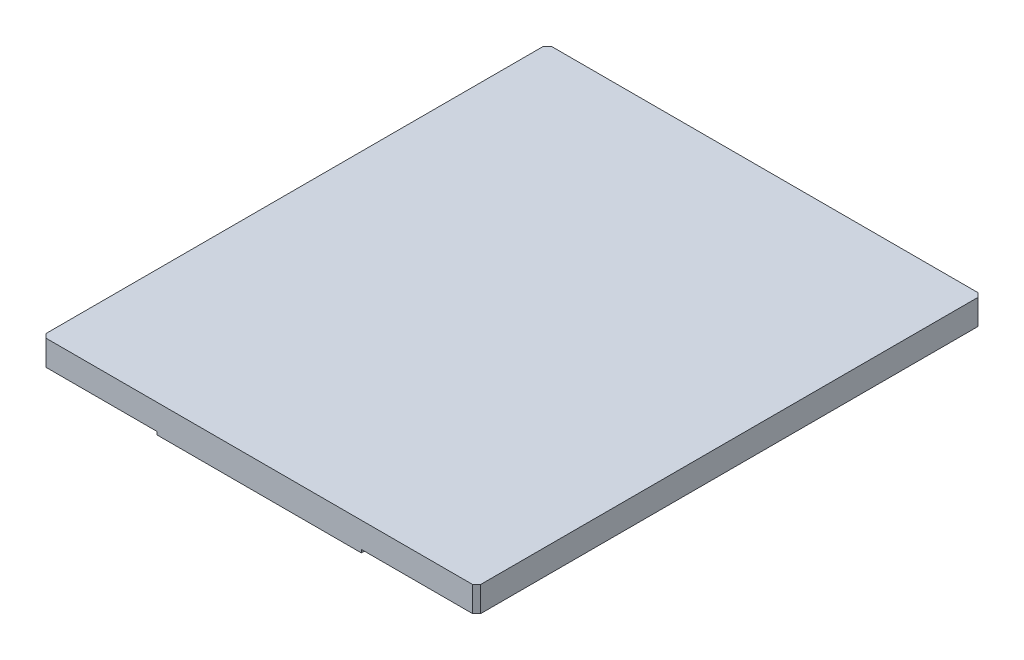
from build123d import *

# Parameters (mm, degrees)
SKETCH_1_W          = 215
SKETCH_1_H          = 250
EXTRUDE_1_DEPTH     = 7
SKETCH_2_W          = 57
SKETCH_2_H          = 250
CUT_EXTRUDE_1_DEPTH = 1.5
CHAMFER_1_SIZE      = 2


with BuildPart() as part:
    # 草图1 → 凸台-拉伸1 (new, symmetric)
    with BuildSketch(Plane(origin=(0, 0, 0), x_dir=(1, 0, 0), z_dir=(0, 1, 0))):
        Rectangle(SKETCH_1_W, SKETCH_1_H)
    extrude(amount=EXTRUDE_1_DEPTH, both=True)

    # 草图2 → 切除-拉伸1 (cut)
    with BuildSketch(Plane.XZ.offset(7)):
        with Locations((79, 0)):
            Rectangle(SKETCH_2_W, SKETCH_2_H)
        with Locations((-79, 0)):
            Rectangle(SKETCH_2_W, SKETCH_2_H)
    extrude(amount=-CUT_EXTRUDE_1_DEPTH, mode=Mode.SUBTRACT)

    # 倒角1
    chamfer_1_edges = [part.edges().sort_by_distance(p)[0] for p in [
        (107.5, 0.75, 125),
        (-107.5, 0.75, 125),
        (-107.5, 0.75, -125),
        (107.5, 0.75, -125),
    ]]
    chamfer(chamfer_1_edges, length=CHAMFER_1_SIZE)


solid = part.part
